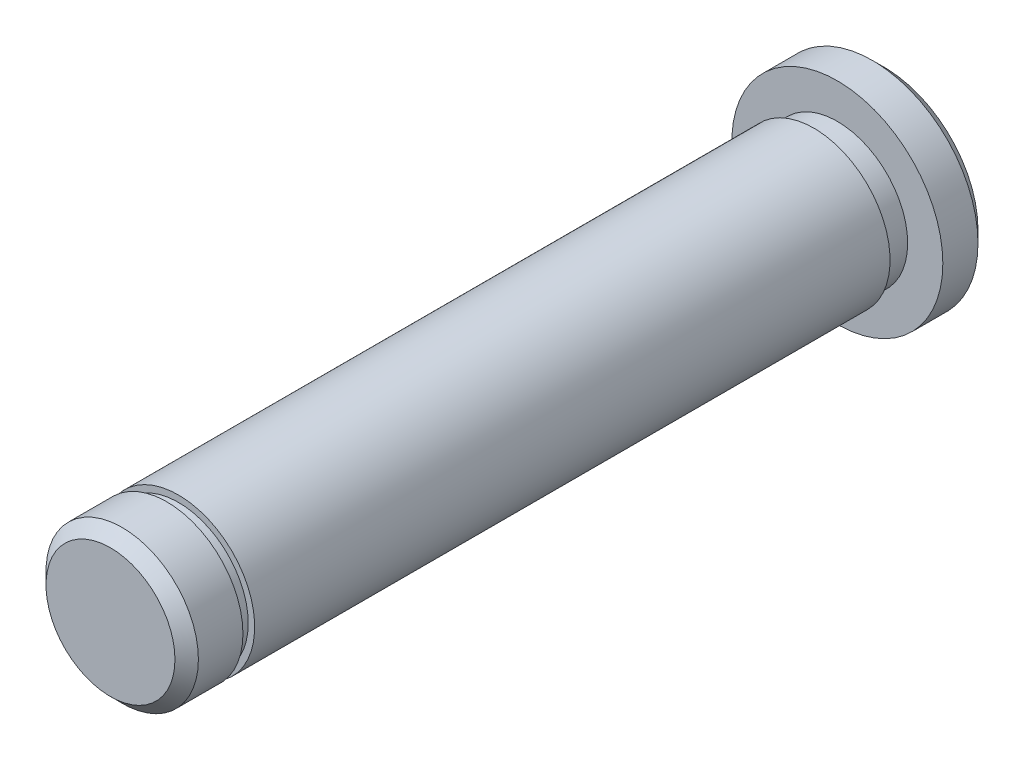
from build123d import *

# Parameters (mm, degrees)
SKETCH1_R           = 9
BOSS_EXTRUDE1_DEPTH = 4
SKETCH2_R           = 6
BOSS_EXTRUDE2_DEPTH = 2
SKETCH3_R           = 6.5
BOSS_EXTRUDE3_DEPTH = 54.2
SKETCH4_R           = 5.95
BOSS_EXTRUDE4_DEPTH = 1
SKETCH5_R           = 6.5
BOSS_EXTRUDE5_DEPTH = 4.8
CHAMFER1_SIZE       = 1


with BuildPart() as part:
    # Sketch1 → Boss-Extrude1 (new body)
    with BuildSketch(Plane.XY):
        Circle(SKETCH1_R)
    extrude(amount=BOSS_EXTRUDE1_DEPTH)

    # Sketch2 → Boss-Extrude2 (add)
    with BuildSketch(Plane.XY.offset(4)):
        Circle(SKETCH2_R)
    extrude(amount=BOSS_EXTRUDE2_DEPTH)

    # Sketch3 → Boss-Extrude3 (add)
    with BuildSketch(Plane.XY.offset(6)):
        with Locations(Location((0, 0, 0), (0, 0, 180))):
            Circle(SKETCH3_R)
    extrude(amount=BOSS_EXTRUDE3_DEPTH)

    # Sketch4 → Boss-Extrude4 (add)
    with BuildSketch(Plane.XY.offset(60.2)):
        Circle(SKETCH4_R)
    extrude(amount=BOSS_EXTRUDE4_DEPTH)

    # Sketch5 → Boss-Extrude5 (add)
    with BuildSketch(Plane.XY.offset(61.2)):
        with Locations(Location((0, 0, 0), (0, 0, 180))):
            Circle(SKETCH5_R)
    extrude(amount=BOSS_EXTRUDE5_DEPTH)

    # Chamfer1
    chamfer1_edges = [part.edges().sort_by_distance(p)[0] for p in [
        (-9, 0, 0),
        (6.5, 0, 66),
    ]]
    chamfer(chamfer1_edges, length=CHAMFER1_SIZE)


solid = part.part
